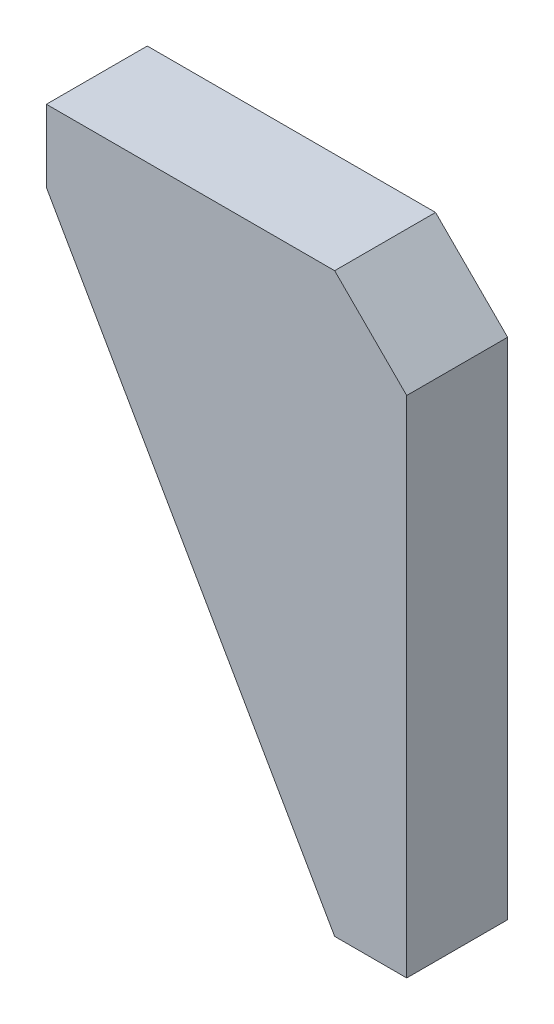
from build123d import *

# Parameters (mm, degrees)
BOSS_EXTRUDE1_DEPTH = 14
CHAMFER1_SIZE       = 10


with BuildPart() as part:
    # Sketch1 → Boss-Extrude1 (new body)
    with BuildSketch(Plane(origin=(0, 0, 0), x_dir=(1, 0, 0), z_dir=(0, 0, -1))):
        Polygon((0, 0), (0, 80), (-10, 80), (-50, 10), (-50, 0), align=None)
    extrude(amount=BOSS_EXTRUDE1_DEPTH)

    # Chamfer1
    chamfer1_edges = [part.edges().sort_by_distance(p)[0] for p in [
        (0, 0, -7),
    ]]
    chamfer(chamfer1_edges, length=CHAMFER1_SIZE)


solid = part.part
